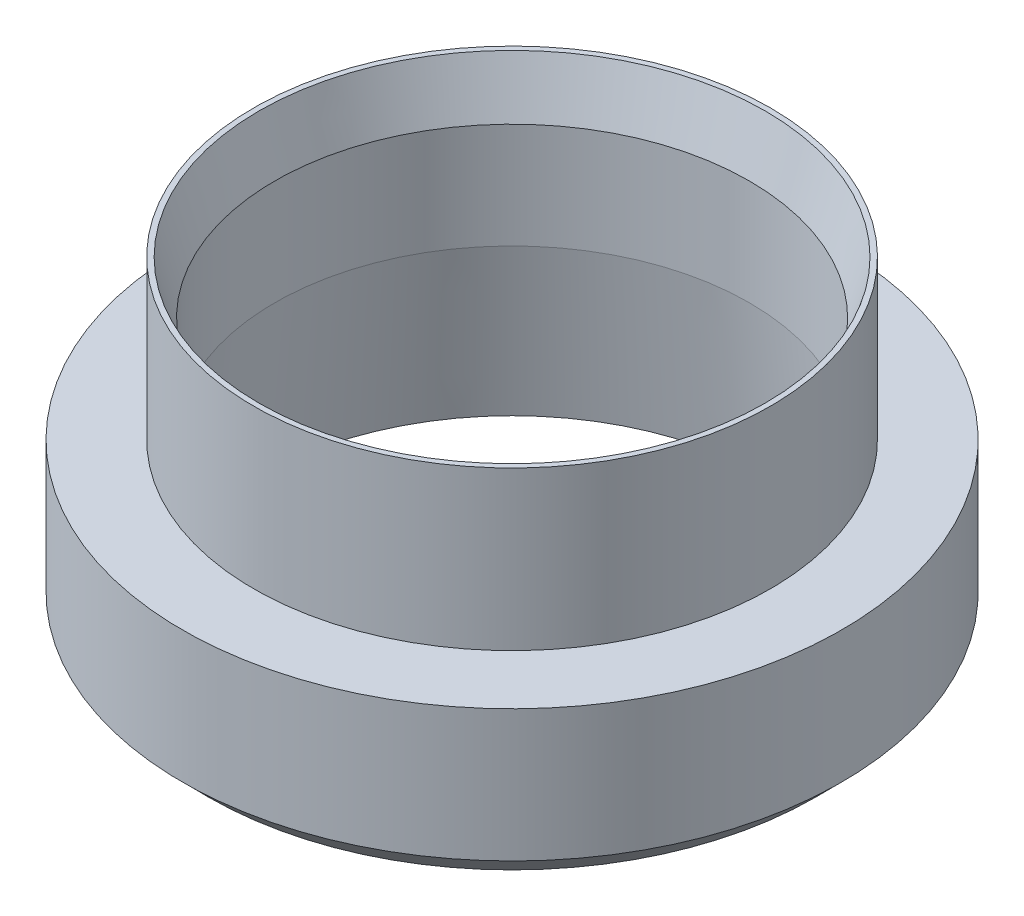
from build123d import *

# Parameters (mm, degrees)
CHAMFER1_SIZE  = 0.5
CHAMFER2_SIZE  = 1
CHAMFER2_SIZE2 = 0.3


with BuildPart() as part:
    # Sketch2 → Revolve1 (revolve)
    with BuildSketch(Plane.XY, mode=Mode.PRIVATE) as revolve1_sk:
        Polygon((4.5, 0), (4.5, 6), (4.9, 6), (4.9, 3), (6.25, 3), (6.25, 0), align=None)
    revolve(revolve1_sk.sketch.rotate(Axis((0, 0, 0), (0, 1, 0)), 90), axis=Axis((0, 0, 0), (0, 1, 0)))

    # Sketch3 → Cut-Revolve1 (revolve, cut)
    with BuildSketch(Plane.XY, mode=Mode.PRIVATE) as cut_revolve1_sk:
        Polygon((4.5, 3), (4.5, 0), (4.8, 0), align=None)
    revolve(cut_revolve1_sk.sketch.rotate(Axis((0, 0, 0), (0, 1, 0)), 90), axis=Axis((0, 0, 0), (0, 1, 0)), mode=Mode.SUBTRACT)

    # Chamfer1
    chamfer1_edges = [part.edges().sort_by_distance(p)[0] for p in [
        (0, 0, 6.25),
    ]]
    chamfer(chamfer1_edges, length=CHAMFER1_SIZE)

    # Chamfer2
    chamfer2_edges = [part.edges().sort_by_distance(p)[0] for p in [
        (0, 6, 4.5),
    ]]
    chamfer2_side = [part.faces().sort_by_distance(p)[0] for p in [
        (0, 4.5, 4.5),
    ]]
    chamfer(chamfer2_edges, length=CHAMFER2_SIZE, length2=CHAMFER2_SIZE2, reference=chamfer2_side[0])


solid = part.part
